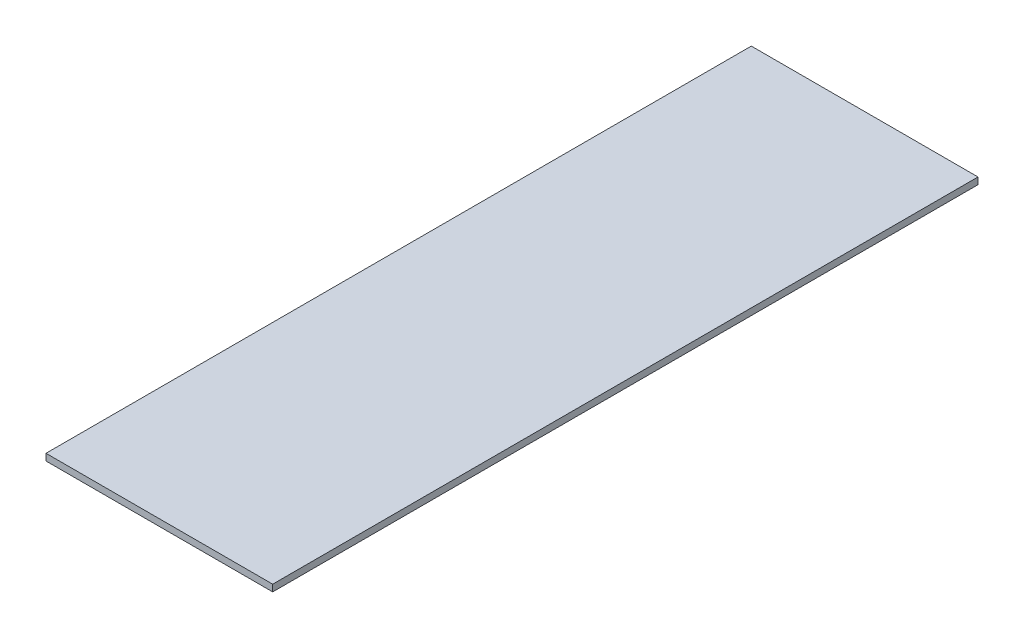
from build123d import *

# Parameters (mm, degrees)
SKETCH1_W           = 135
SKETCH1_H           = 420
BOSS_EXTRUDE1_DEPTH = 4


with BuildPart() as part:
    # Sketch1 → Boss-Extrude1 (new body)
    with BuildSketch(Plane(origin=(0, 0, 0), x_dir=(1, 0, 0), z_dir=(0, 1, 0))):
        Rectangle(SKETCH1_W, SKETCH1_H)
    extrude(amount=BOSS_EXTRUDE1_DEPTH)


solid = part.part
